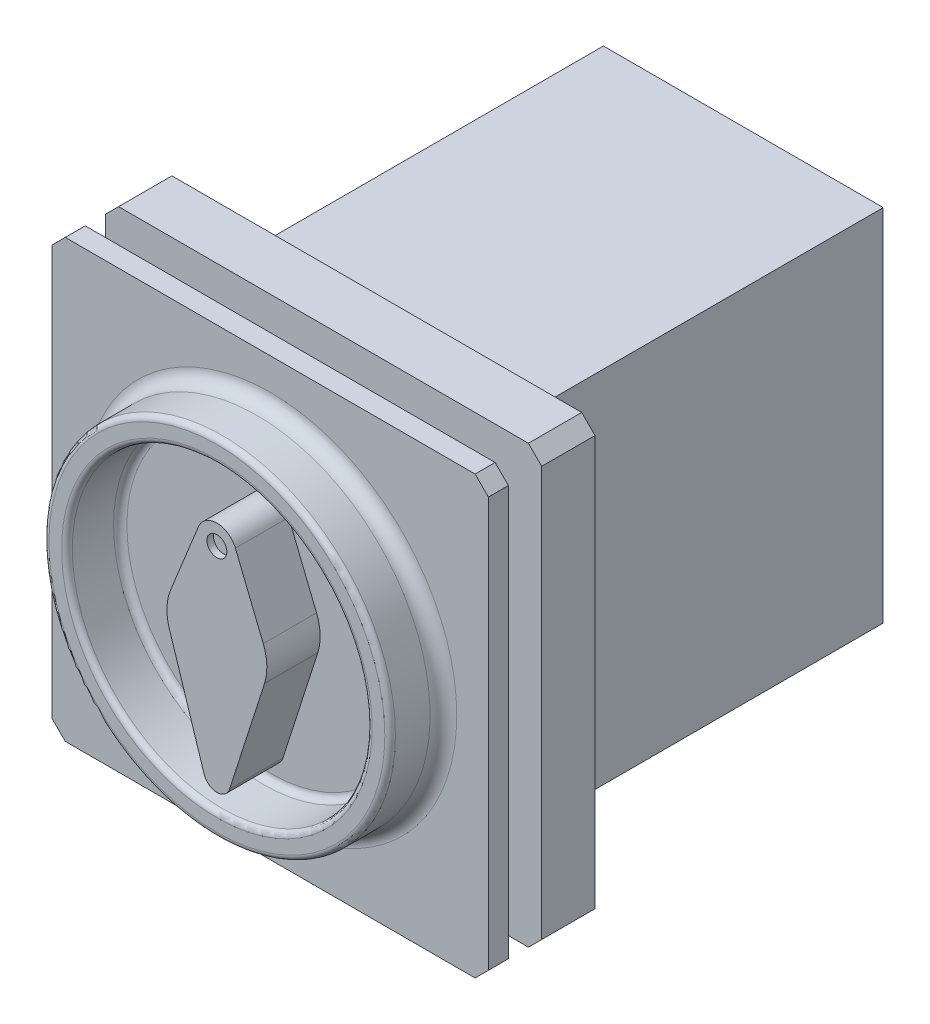
SolidWorks part; units mm, degrees
ref_plane "前视" through (0, 0, 0) normal (0, 0, 1) x (1, 0, 0)
ref_plane "上视" through (0, 0, 0) normal (0, 1, 0) x (1, 0, 0)
ref_plane "右视" through (0, 0, 0) normal (1, 0, 0) x (0, 0, -1)
sketch "草图1" plane through (0, 0, 0) normal (0, 0, 1) x (1, 0, 0)
  line L1 (-21, -27) -> (21, -27)
  line L2 (-21, -27) -> (-21, 27)
  line L3 (-21, 27) -> (21, 27)
  line L4 (21, -27) -> (21, 27)
  line L5 (-21, -27) -> (21, 27) construction
  line L6 (-21, 27) -> (21, -27) construction
  point P0 (0, 0)
  dimension "D1" = 42
  dimension "D2" = 54
extrude "凸台-拉伸1" add sketch "草图1" along normal blind 55
sketch "草图5" plane through (0, 0, 55) normal (0, 0, 1) x (1, 0, 0)
  line L1 (-32.75, -32.75) -> (32.75, -32.75)
  line L2 (-32.75, -32.75) -> (-32.75, 32.75)
  line L3 (-32.75, 32.75) -> (32.75, 32.75)
  line L4 (32.75, -32.75) -> (32.75, 32.75)
  line L5 (-32.75, -32.75) -> (32.75, 32.75) construction
  line L6 (-32.75, 32.75) -> (32.75, -32.75) construction
  point P0 (0, 0)
  dimension "D1" = 65.5
extrude "凸台-拉伸3" add sketch "草图5" along normal blind 8
sketch "草图6" plane through (0, 0, 63) normal (0, 0, 1) x (1, 0, 0)
  circle A0 centre (0, 0) radius 10
  dimension "D1" = 20
extrude "凸台-拉伸4" add sketch "草图6" along normal blind 5
hole_wizard "M4 螺纹孔1" positions "草图8" profile "草图7" tap size "M4" standard "Iso"
sketch "草图8" plane through (0, 0, 63) normal (0, 0, 1) x (1, 0, 0)
  line L0 (-24, 24) -> (24, 24) construction
  line L1 (24, 24) -> (24, -24) construction
  line L3 (0, 24) -> (0, 0) construction
  line L4 (0, 0) -> (24, 0) construction
  point P0 (-24, 24)
  point P2 (24, 24)
  point P4 (24, -24)
  point P6 (-24, -24)
  dimension "D1" = 48
sketch "草图7" plane through (-24, 24, 63) normal (1, 0, 0) x (0, -1, 0)
  line L0 (0, 0) -> (0, 12.4914)
  line L1 (0, 12.4914) -> (1.65, 11.5)
  line L2 (1.65, 11.5) -> (1.65, 0)
  line L5 (1.65, 0) -> (0, 0)
  line L10 (0, 12.4914) -> (-1.65, 11.5) construction
  line L11 (0, -6.35) -> (0, 107.95) construction
  dimension "螺纹孔钻头直径" = 3.3
  dimension "螺纹孔钻头深度" = 11.5
  dimension "导头角度" = 118
cosmetic thread "孔螺蚊线1" parameters "D1"=8, "D2"=4
cosmetic thread "孔螺蚊线2" parameters "D1"=8, "D2"=4
cosmetic thread "孔螺蚊线3" parameters "D1"=8, "D2"=4
cosmetic thread "孔螺蚊线4" parameters "D1"=8, "D2"=4
chamfer "倒角1" distance 2 angle 45 4 edges at (32.75, -32.75, 59) (-32.75, -32.75, 59) (-32.75, 32.75, 59) (32.75, 32.75, 59)
sketch "草图9" plane through (0, 0, 68) normal (0, 0, 1) x (1, 0, 0)
  line L0 (32.75, -30.75) -> (32.75, 30.75) construction
  line L1 (-32.75, -32.75) -> (32.75, -32.75)
  line L2 (-32.75, -32.75) -> (-32.75, 32.75)
  line L3 (-32.75, 32.75) -> (32.75, 32.75)
  line L4 (32.75, -32.75) -> (32.75, 32.75)
  line L5 (-32.75, -32.75) -> (32.75, 32.75) construction
  line L6 (-32.75, 32.75) -> (32.75, -32.75) construction
  line L8 (30.75, 32.75) -> (-30.75, 32.75) construction
  point P0 (0, 0)
extrude "凸台-拉伸5" add sketch "草图9" along normal blind 3
sketch "草图10" plane through (0, 0, 71) normal (0, 0, 1) x (1, 0, 0)
  circle A0 centre (0, 0) radius 26
  circle A1 centre (0, 0) radius 22.5
  dimension "D1" = 52
  dimension "D2" = 45
extrude "凸台-拉伸6" add sketch "草图10" along normal blind 8
sketch "草图11" plane through (0, 0, 71) normal (0, 0, 1) x (1, 0, 0)
  line L0 (0, 12) -> (0, 0) construction
  line L1 (0, 0) -> (0, -18) construction
  line L2 (2.7811, 13.125) -> (6.9527, 2.8125)
  line L3 (7.1413, -2.2917) -> (1.9043, -18.6111)
  line L4 (-7.1413, -2.2917) -> (-1.9043, -18.6111)
  line L5 (-2.7811, 13.125) -> (-6.9527, 2.8125)
  arc A0 (-6.9527, 2.8125) -> (-7.1413, -2.2917) centre (0, 0) ccw
  arc A1 (2.7811, 13.125) -> (-2.7811, 13.125) centre (0, 12) ccw
  arc A2 (-1.9043, -18.6111) -> (1.9043, -18.6111) centre (0, -18) ccw
  arc A3 (7.1413, -2.2917) -> (6.9527, 2.8125) centre (0, 0) ccw
  dimension "D1" = 15
  dimension "D4" = 4
  dimension "D5" = 6
  dimension "D2" = 18
  dimension "D3" = 12
extrude "凸台-拉伸7" add sketch "草图11" along normal up to surface (8 mm away) up to face at (26, 0, 79)
fillet "圆角1" radius 2 1 edges at (-26, 0, 71)
fillet "圆角2" radius 1 1 edges at (22.5, 0, 71)
fillet "圆角3" radius 0.8 2 edges at (22.5, 0, 79) (26, 0, 79)
sketch "草图12" plane through (0, 0, 79) normal (0, 0, 1) x (1, 0, 0)
  circle A0 centre (0, 12) radius 1.5
  arc A1 (2.7811, 13.125) -> (-2.7811, 13.125) centre (0, 12) ccw construction
  dimension "D1" = 3
extrude "切除-拉伸1" cut sketch "草图12" against normal blind 1
chamfer "倒角2" distance 2 angle 45 4 edges at (32.75, -32.75, 69.5) (-32.75, -32.75, 69.5) (-32.75, 32.75, 69.5) (32.75, 32.75, 69.5)
